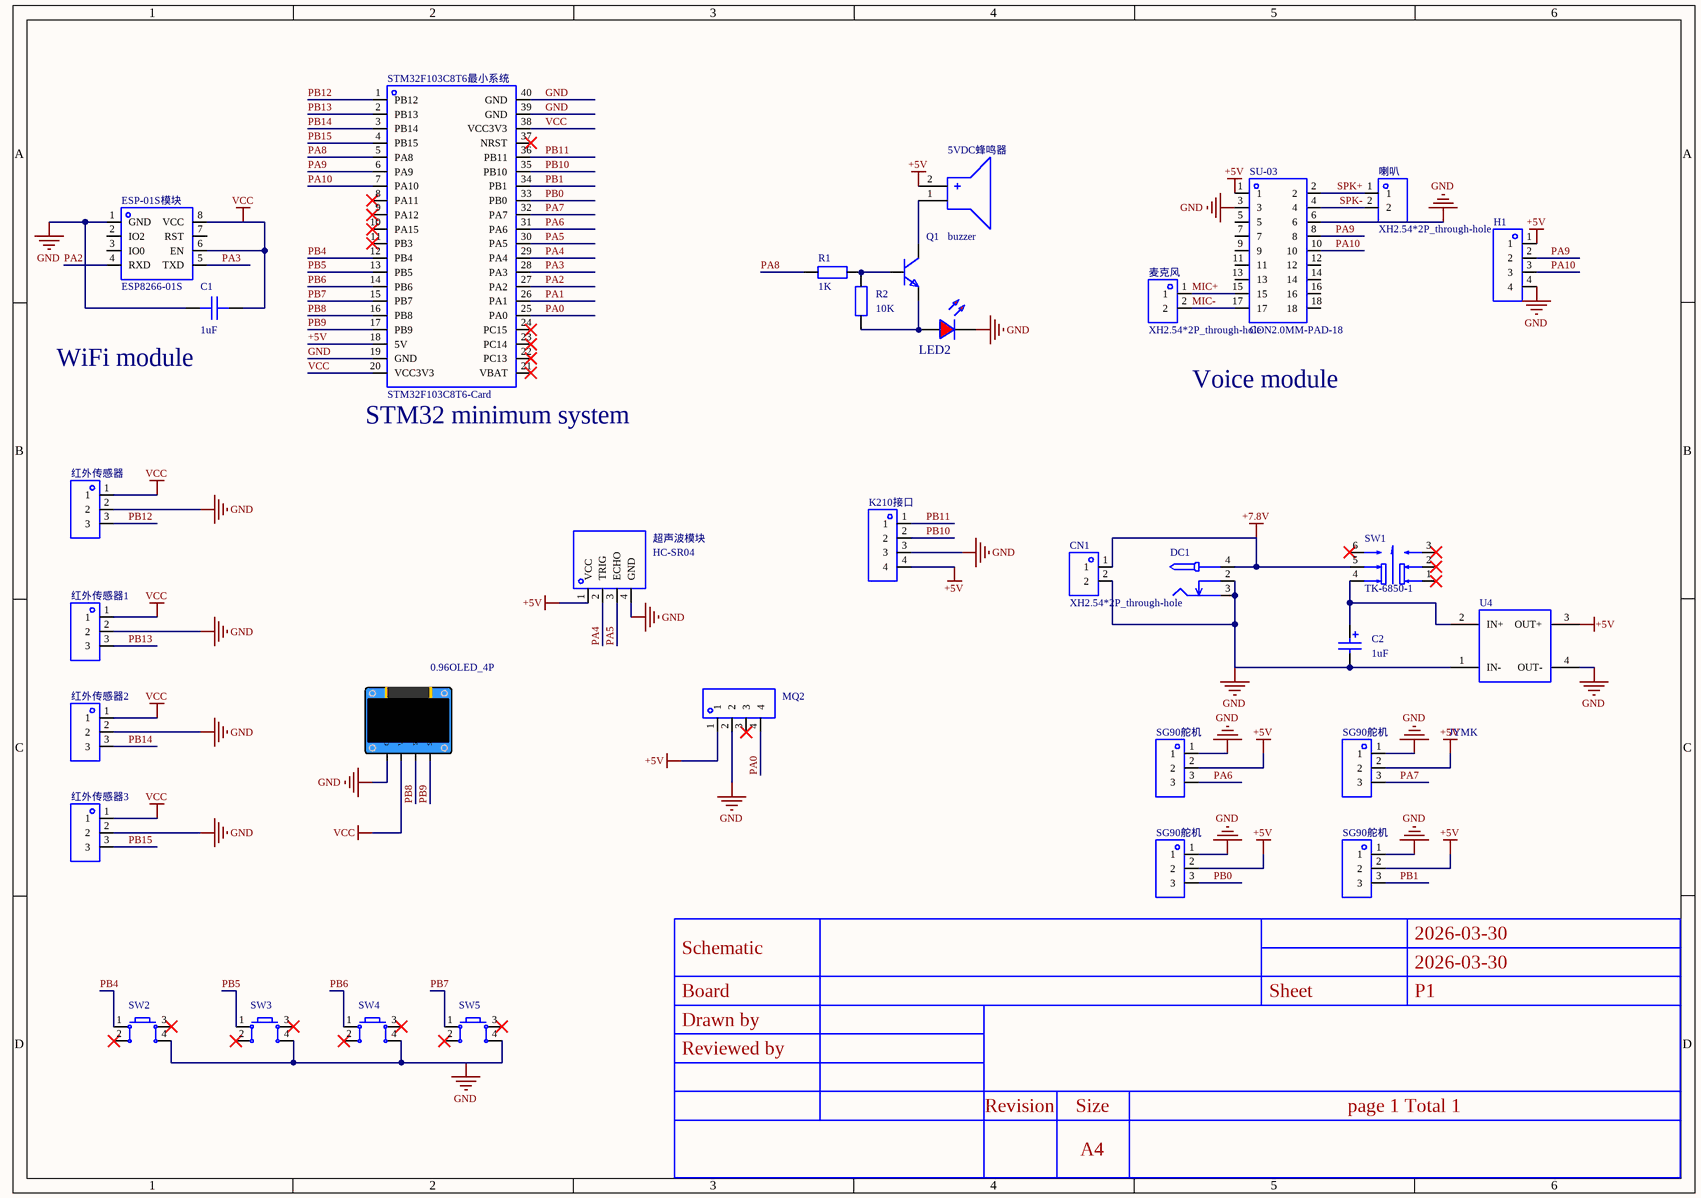
[diagram p0: MISC89030-3.schdoc]
# Altium project MISC89030-2.PrjPcb
1 sheet, 33 parts. Net scope: global (net labels, ports and power ports of the same name join across sheets).
Board file: MISC89030.pcbdoc

## Sheet MISC89030-3.schdoc
size 297 x 209 mm; Version: V1.0; @Project Name: MISC89030; @Page Count: 1; @Update Date: 2026-03-30; @Create Date: 2026-03-30; @Schematic Name: MISC89030; @Page No: 1; @Create Time: 18:58:15; @Update Time: 22:44:58; @Board Name: MISC89030

### Parts
(Parts that share a designator on the sheet are numbered #1, #2 ... from top to bottom, then left to right.)
0.96OLED_4P  (no value)  [0.96OLED_4P]
5VDC蜂鸣器  buzzer  [BUZ-TH_BD12.0-P6.00-D0.9-RD]
C1  1uF  [C0603]
C2  1uF  [C_Ele_SMD_3x5.4mm]
CN1  XH2.54*2P_through-hole  [CONN-TH_2P-P2.50-XH2.54-2P]
DC1  (no value)  [DC-2.0]
ESP-01S模块  ESP8266-01S  [WIFIM-TH_ESP8266-01S]
H1  (no value)  [HDR-TH_4P-P2.54-V-M]
K210接口  (no value)  [HDR-TH_4P-P2.54-V-F]
LED2  (no value)  [LED_0603]
MQ2  (no value)  [HDR-TH_4P-P2.54-V-F]
Q1  (no value)  [S8050_SOT-23]
R1  1K  [R0603]
R2  10K  [R0603]
SG90舵机#1  (no value)  [HDR-TH_3P-P2.54-V-F]
SG90舵机#2  (no value)  [HDR-TH_3P-P2.54-V-F]
SG90舵机#3  (no value)  [HDR-TH_3P-P2.54-V-F]
SG90舵机#4  (no value)  [HDR-TH_3P-P2.54-V-F]
STM32F103C8T6最小系统  STM32F103C8T6-Card  [CONN-TH_L53.3-W22.9_STM32F103C8T6-CARD]
SU-03  CON2.0MM-PAD-18  [CONN-TH_18P-P2.00_C9900078766]
SW1  TK-6850-1  [SW-TH_TK-6850-1]
SW2  (no value)  [SW-TH_4P-L6.0-W6.0-P4.50-LS6.5]
SW3  (no value)  [SW-TH_4P-L6.0-W6.0-P4.50-LS6.5]
SW4  (no value)  [SW-TH_4P-L6.0-W6.0-P4.50-LS6.5]
SW5  (no value)  [SW-TH_4P-L6.0-W6.0-P4.50-LS6.5]
U4  (no value)  [JYMK]
喇叭  XH2.54*2P_through-hole  [CONN-TH_2P-P2.50-XH2.54-2P]
红外传感器  (no value)  [HDR-TH_3P-P2.54-V-F]
红外传感器1  (no value)  [HDR-TH_3P-P2.54-V-F]
红外传感器2  (no value)  [HDR-TH_3P-P2.54-V-F]
红外传感器3  (no value)  [HDR-TH_3P-P2.54-V-F]
超声波模块  HC-SR04  [TH_HC-SR04V]
麦克风  XH2.54*2P_through-hole  [CONN-TH_2P-P2.50-XH2.54-2P]

### Nets
+5V: 5VDC蜂鸣器.2(+) H1.1 K210接口.4 MQ2.1 SG90舵机#1.2 SG90舵机#2.2 SG90舵机#3.2 SG90舵机#4.2 STM32F103C8T6最小系统.18(5V) SU-03.1 U4.3(OUT+) 超声波模块.1(VCC)
+7.8V: CN1.1 DC1.4 SW1.5
GND: 0.96OLED_4P.1(GND) C1.1 C2.2 CN1.2 DC1.2 DC1.3 ESP-01S模块.1(GND) H1.4 K210接口.3 LED2.1(C) MQ2.2 SG90舵机#1.1 SG90舵机#2.1 SG90舵机#3.1 SG90舵机#4.1 STM32F103C8T6最小系统.19(GND) STM32F103C8T6最小系统.39(GND) STM32F103C8T6最小系统.40(GND) SU-03.3 SU-03.6 SW2.4 SW3.4 SW4.4 SW5.4 U4.1(IN-) U4.4(OUT-) 红外传感器.2 红外传感器1.2 红外传感器2.2 红外传感器3.2 超声波模块.4(GND)
VCC: 0.96OLED_4P.2(VCC) C1.2 ESP-01S模块.6(EN) ESP-01S模块.8(VCC) STM32F103C8T6最小系统.20(VCC3V3) STM32F103C8T6最小系统.38(VCC3V3) 红外传感器.1 红外传感器1.1 红外传感器2.1 红外传感器3.1
MIC+: SU-03.15 麦克风.1
MIC-: SU-03.17 麦克风.2
PA0: MQ2.4 STM32F103C8T6最小系统.25(PA0)
PA1: STM32F103C8T6最小系统.26(PA1)
PA2: ESP-01S模块.4(RXD) STM32F103C8T6最小系统.27(PA2)
PA3: ESP-01S模块.5(TXD) STM32F103C8T6最小系统.28(PA3)
PA4: STM32F103C8T6最小系统.29(PA4) 超声波模块.2(TRIG)
PA5: STM32F103C8T6最小系统.30(PA5) 超声波模块.3(ECHO)
PA6: SG90舵机#1.3 STM32F103C8T6最小系统.31(PA6)
PA7: SG90舵机#2.3 STM32F103C8T6最小系统.32(PA7)
PA8: R1.1 STM32F103C8T6最小系统.5(PA8)
PA9: H1.2 STM32F103C8T6最小系统.6(PA9) SU-03.8
PA10: H1.3 STM32F103C8T6最小系统.7(PA10) SU-03.10
PB0: SG90舵机#3.3 STM32F103C8T6最小系统.33(PB0)
PB1: SG90舵机#4.3 STM32F103C8T6最小系统.34(PB1)
PB4: STM32F103C8T6最小系统.12(PB4) SW2.1
PB5: STM32F103C8T6最小系统.13(PB5) SW3.1
PB6: STM32F103C8T6最小系统.14(PB6) SW4.1
PB7: STM32F103C8T6最小系统.15(PB7) SW5.1
PB8: 0.96OLED_4P.3(SCL) STM32F103C8T6最小系统.16(PB8)
PB9: 0.96OLED_4P.4(SDA) STM32F103C8T6最小系统.17(PB9)
PB10: K210接口.2 STM32F103C8T6最小系统.35(PB10)
PB11: K210接口.1 STM32F103C8T6最小系统.36(PB11)
PB12: STM32F103C8T6最小系统.1(PB12) 红外传感器.3
PB13: STM32F103C8T6最小系统.2(PB13) 红外传感器1.3
PB14: STM32F103C8T6最小系统.3(PB14) 红外传感器2.3
PB15: STM32F103C8T6最小系统.4(PB15) 红外传感器3.3
SPK+: SU-03.2 喇叭.1
SPK-: SU-03.4 喇叭.2
Net5VDC蜂鸣器_1: 5VDC蜂鸣器.1(-) Q1.3
NetC2_1: C2.1 SW1.4 U4.2(IN+)
NetLED2_2: LED2.2(A) Q1.2 R2.1
NetQ1_1: Q1.1 R1.2 R2.2

Not connected (* = marked no-connect by the designer): ESP-01S模块 2(IO2) 3(IO0) 7(RST); MQ2 3*; STM32F103C8T6最小系统 8(PA11)* 9(PA12)* 10(PA15)* 11(PB3)* 21(VBAT)* 22(PC13)* 23(PC14)* 24(PC15)* 37(NRST)*; SU-03 5 7 9 11 12 13 14 16 18; SW1 1* 2* 3* 6*; SW2 2* 3*; SW3 2* 3*; SW4 2* 3*; SW5 2* 3*

### Notes on the sheet
- (near C1) WiFi module
- (near STM32F103C8T6最小系统) STM32 minimum system
- Voice module
- 2026-03-30
- Schematic
- Board
- Sheet
- P1
- Drawn by
- Reviewed by
- Revision
- Size
- A4
- page 1 Total 1

### Library data of the parts
0.96OLED_4P = 0.96OLED模块_4P: Symbol: 0.96OLED module_4P; ConvertToPcb: yes; ModelId: 79c000fdb68d45a296c2e9bedf4f9055; ModelTransform: 1393.69792,1318.895,0,0,0,0,0,-560.079,-137.795; Device: 0.96OLED module_4P; AddInBom: yes; FootprintName: 0.96OLED_4P; Supplier Footprint: 插件; ModelName: 0.96OLED_4P
5VDC蜂鸣器 = buzzer: AddInBom: yes; ModelId: af17e4151ed84fc2a628230bf23763630819f05c4eef4c71ace90d822a990e87; ModelTransform: 472.44,472.176,0,270,0,0,0,0,-196.85; Symbol: BUZZER; Device: buzzer; LCSC Part Name: buzzer; SupplierPart: C9900014030; ManufacturerPart: buzzer; Supplier Footprint: buzzer; JLCPCB Part Class: Extended Part; Supplier: LCSC; ConvertToPcb: yes; FootprintName: BUZ-TH_BD12.0-P6.00-D0.9-RD; ModelName: BUZ-TH_BD12.0-P6.00-D0.9-RD
C1 = CAP_0603: Symbol: Capacitance; ConvertToPcb: yes; ModelId: ac125912035d415993ca9572d50418b10819f05c4eef4c71ace90d822a990e87; ModelName: C0603_L1.6-W0.8-H0.8; ModelTransform: 62.992,31.496,0,0,0,0,0,0,0; Device: CAP_0603; Value: 1uF; AddInBom: yes; Supplier Footprint: 0603; FootprintName: C0603
C2 = C_Ele_SMD_3x5.4mm: Symbol: CAP; AddInBom: yes; ModelId: 0132c3d3fdbf4fd987f710a97e7a5b5d; ModelName: CAP-SMD_BD3.0-L3.3-W3.3-H5.3; ModelTransform: 129.9,149.58,209.06,-90,0,0,0,0,0; Device: C_Ele_SMD_3x5.4mm; Value: 1uF; Supplier Footprint: SMD,3x5.4mm; ConvertToPcb: yes; FootprintName: C_Ele_SMD_3x5.4mm
CN1 喇叭 麦克风 = XH2.54*2P_直插: 3D Model: 325c595e30db4df8abe76612dd40b0fa0819f05c4eef4c71ace90d822a990e87; 3D Model Transform: 295.275,228.346,0,180,0,0,-0.002,-20.079,-137.795; AddInBom: yes; Symbol: XH2.54*2P_through-hole; Device: XH2.54*2P_through-hole; LCSC Part Name: XH2.54*2P_直插; Supplier Part: C9900008615; Manufacturer Part: XH2.54*2P_直插; Supplier Footprint: XH2.54_2P; JLCPCB Part Class: Extended Part; Supplier: LCSC; ConvertToPcb: yes; FootprintName: CONN-TH_2P-P2.50-XH2.54-2P; ModelName: CONN-TH_2P-P2.50-XH2.54-2P
DC1 = DC-005_2.0: Symbol: DC power jack; ConvertToPcb: yes; ModelId: f5f20b8a2308479b936ba3c2698865bb0819f05c4eef4c71ace90d822a990e87; ModelName: DC-IN-TH_DC-5520-1; ModelTransform: 372.05,551.18,582.68,90,0,0,137.8,0,-149.61; Device: DC-005_2.0; AddInBom: yes; Supplier Footprint: 插件; FootprintName: DC-2.0
ESP-01S模块 = ESP8266-01S: AddInBom: yes; ModelId: 7671a3a19d0d4245ae5d5806b59f4d510819f05c4eef4c71ace90d822a990e87; ModelTransform: 566.928,972.439,0,0,0,0,0,378.464,-118.11; Symbol: ESP8266-01S; Device: ESP8266-01S; LCSC Part Name: ESP8266-01S; SupplierPart: C9900150497; ManufacturerPart: ESP8266-01S; Supplier Footprint: TH-8P; JLCPCB Part Class: Extended Part; Supplier: LCSC; ConvertToPcb: yes; FootprintName: WIFIM-TH_ESP8266-01S; ModelName: WIFIM-TH_ESP8266-01S
H1 = HDR-M_2.54_1x4P: Symbol: PZ254V-11-04P; ConvertToPcb: yes; ModelId: 112f4d05e8d64e99ab9a333894bea4f90819f05c4eef4c71ace90d822a990e87; ModelName: HDR-TH_4P-P2.54-M-LI-1X4P; ModelTransform: 399.999,104.7242,0,0,0,0,0,0,-118.11; Device: HDR-M_2.54_1x4P; AddInBom: yes; SupplierPart: C492403; Supplier Footprint: 插件; FootprintName: HDR-TH_4P-P2.54-V-M
K210接口 MQ2 = HDR-F_2.54_1x4P: Symbol: 2.54-1*4P female; 3D Model: d187812051054f85879fcaa51a310d8e0819f05c4eef4c71ace90d822a990e87; 3D Model Transform: 419.6842,98.464,0,0,0,0,0,0,-118.11; ConvertToPcb: yes; Device: HDR-F_2.54_1x4P; Supplier Part: C2718488; Supplier Footprint: 插件; AddInBom: yes; FootprintName: HDR-TH_4P-P2.54-V-F; ModelName: HDR-TH_4P-P2.54-V-F
LED2 = LED_0603-R: Symbol: LED_R; Convert to PCB: yes; 3D Model: dd8257b0d61a4cd7b68939a056e08095; 3D Model Transform: 58.72,29.4,22.03,0,0,0,0,0,0; ModelName: LED-0603_R; Device: LED_0603-R; Add into BOM: yes; Supplier Footprint: 0603; FootprintName: LED_0603
Q1 = S8050_SOT_NPN: Symbol: NPN; ConvertToPcb: yes; ModelId: c62791f0466c4ae2a892c056b845b0ca0819f05c4eef4c71ace90d822a990e87; ModelName: SOT-23-3P_L2.9-W1.3-H1.0-LS2.4-P0.95; ModelTransform: 98.6,114.12,41.29,180,0,0,0,0,-3; Device: S8050_SOT_NPN; AddInBom: yes; Supplier Footprint: SOT-23; FootprintName: S8050_SOT-23
R1 R2 = Res_0603: Symbol: Resistor; ConvertToPcb: yes; ModelId: fc143cca1e79419f9cd78b61e9279f080819f05c4eef4c71ace90d822a990e87; ModelTransform: 31.8897,63.7794,0,90,0,0,0,0,0; Device: Res_0603; AddInBom: yes; Supplier Footprint: 0603; FootprintName: R0603; ModelName: R0603
  R1: Value: 1K
  R2: Value: 10K
SG90舵机#1-SG90舵机#4 红外传感器 红外传感器1-红外传感器3 = HDR-F_2.54_1x3P: Symbol: PM254V-11-03-H85; 3D Model: f3b3cc5aae9641bf9e56fc160cef875b; 3D Model Transform: 299.9994,100,0,0,0,0,0,0,-118.11; ConvertToPcb: yes; ModelName: HDR2.54-F-LI-1X3P; Device: HDR-F_2.54_1x3P; Supplier Part: C541850; Supplier Footprint: 插件; AddInBom: yes; FootprintName: HDR-TH_3P-P2.54-V-F
STM32F103C8T6最小系统 = STM32F103C8T6-Card: AddInBom: yes; Symbol: STM32F103C8T6-CARD; Device: STM32F103C8T6-Card; LCSC Part Name: STM32F103C8T6-Card; SupplierPart: C9900077949; ManufacturerPart: STM32F103C8T6-Card; Supplier Footprint: 插件; Supplier: LCSC; ConvertToPcb: yes; FootprintName: CONN-TH_L53.3-W22.9_STM32F103C8T6-CARD
SU-03 = CON2.0MM-PAD-18: 3D Model: 07100c6dd3a4442ea12d6f5a4e41c4c80819f05c4eef4c71ace90d822a990e87; 3D Model Transform: 787.7937,374.015,0,0,0,0,0,-14.961,-118.11; AddInBom: yes; Symbol: CON2.0MM-PAD-18; Device: CON2.0MM-PAD-18; LCSC Part Name: CON2.0MM-PAD-18; Supplier Part: C9900078766; Manufacturer Part: CON2.0MM-PAD-18; Supplier Footprint: TH-2*9P-2.0; JLCPCB Part Class: Extended Part; Supplier: LCSC; ConvertToPcb: yes; FootprintName: CONN-TH_18P-P2.00_C9900078766; ModelName: CONN-TH_18P-P2.00_C9900078766
SW1 = TK-6850-1: Circuit structure: DPDT; Self-lock/no-lock: self-lock; Mounting type: through-hole; Operating force: 2.4N; Operating life: -;; Manufacturer: Yuandi(元迪); AddInBom: yes; ModelId: 80b2f56b51c94ac4847e8b4c36c572b70819f05c4eef4c71ace90d822a990e87; ModelTransform: 342.519,334.645,0,0,0,0,-3.937,0,-137.795; Actuator Style: Rectangular plunger; Actuator/Cap Color: White; Symbol: TK-6850-1; Device: TK-6850-1; LCSC Part Name: 自锁开关8.5*8.5*13.8有声有锁高导高柄插件双排6P按键开关带锁DIP六脚; SupplierPart: C528790; ManufacturerPart: TK-6850-1; Supplier Footprint: 插件; JLCPCB Part Class: Extended Part; Datasheet: example.com/datasheet/TK-6850-1/548579.html; Supplier: LCSC; ConvertToPcb: yes; FootprintName: SW-TH_TK-6850-1; ModelName: SW-TH_TK-6850-1; Circuit: DPDT; Self Lock / No Lock: Self-lock; Mounting Type: Through-hole; Termination Style: PC pin; Operating Force: 2.4N; Life: -
SW2-SW5 = Key_TH_6x6x6: Contact current: 50mA; Rated voltage (DC): 12V; Insulation resistance: 100MΩ; Circuit structure: SPST; Mounting type: through-hole; Button shape: round button; Button/cap color: black; Operating force: 260gf@±30gf; Operating temperature: -25℃~+70℃; Pin style: PC pin; Switch length: 6mm; Switch width: 6mm; Switch height: 6mm; With bracket: no;; Symbol: Tactile switch; AddInBom: yes; ModelId: 20eee248bc684ccd8cbdbb1d0d91ec6f0819f05c4eef4c71ace90d822a990e87; ModelName: SW-TH_4P-L6.0-W6.0-H5.0-LS6.5-P4.50; ModelTransform: 236.22,323.03,0,90,0,0,0,0,-137.795; Device: Key_TH_6x6x6; ConvertToPcb: yes; FootprintName: SW-TH_4P-L6.0-W6.0-P4.50-LS6.5; Supplier Footprint: 插件
U4 = JYMK: Convert to PCB: yes; Symbol: JYMK; Device: JYMK; AddInBom: yes; FootprintName: JYMK
超声波模块 = HC-SR04: Manufacturer: Universal Microelectronics; AddInBom: yes; Symbol: HC-SR04; Device: HC-SR04; LCSC Part Name: HC-SR04; SupplierPart: C19857336; ManufacturerPart: HC-SR04; Supplier Footprint: -; JLCPCB Part Class: Extended Part; Datasheet: example.com/datasheet/HC-SR04/21184790.html; Supplier: LCSC; ConvertToPcb: yes; FootprintName: TH_HC-SR04V